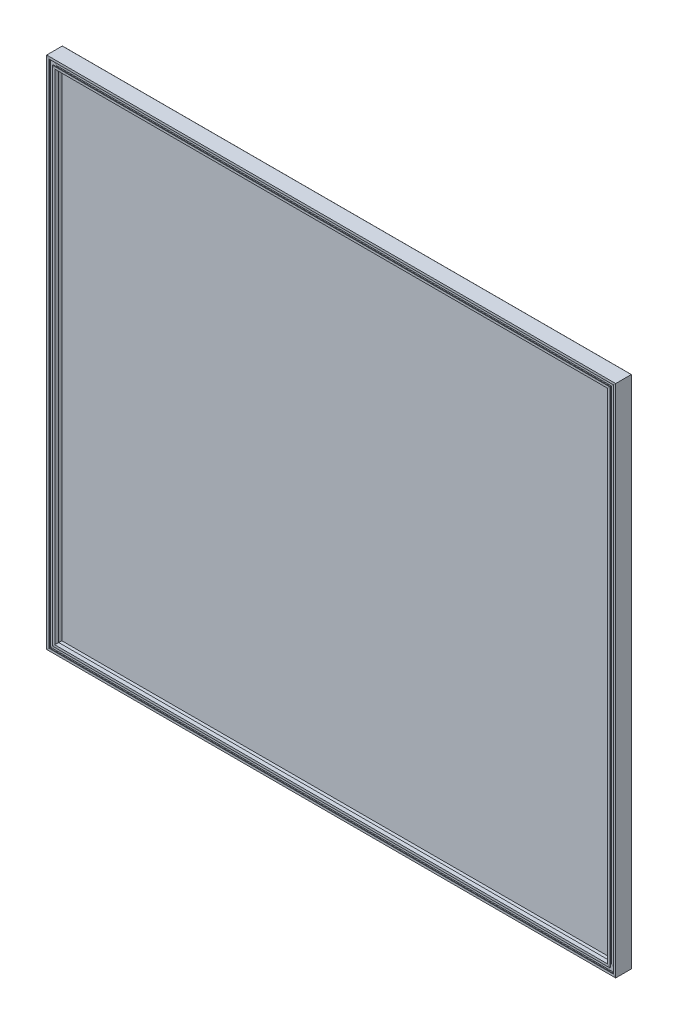
from build123d import *

# Parameters (mm, degrees)
MEMBER_1_DEPTH      = 40.357337308
MEMBER_1_DEPTH_BACK = 1300.357337308
MEMBER_1_2_DEPTH    = 1220.714674617
MEMBER_1_3_DEPTH    = 1340.714674617
MEMBER_1_4_DEPTH    = 1220.714674617
SKETCH_12_W         = 1250
SKETCH_12_H         = 1130
EXTRUDE_1_DEPTH     = 3


with BuildPart() as part:
    # 草图11 → Member 1 (new, two sides: drawn at the far end of the back side and taken through both)
    with BuildSketch(Plane(origin=(-630, 570, 0), x_dir=(0, -1, 0), z_dir=(-1, 0, 0)).offset(-MEMBER_1_DEPTH_BACK)):
        with BuildLine():
            Line((13, -1.5), (13, 0))
            Line((13, 0), (18, 0))
            Line((18, 0), (18, -8.7))
            Line((18, -8.7), (2, -8.7))
            Line((2, -8.7), (2, -32))
            ThreePointArc((2, -32), (2.292893219, -32.707106781), (3, -33))
            Line((3, -33), (8, -33))
            Line((8, -33), (8, -31.5))
            Line((8, -31.5), (10, -31.5))
            Line((10, -31.5), (10, -35))
            Line((10, -35), (0.5, -35))
            ThreePointArc((0.5, -35), (0.146446609, -34.853553391), (0, -34.5))
            Line((0, -34.5), (0, 0))
            Line((0, 0), (5, 0))
            Line((5, 0), (5, -1.5))
            Line((5, -1.5), (2, -1.5))
            Line((2, -1.5), (2, -6.7))
            Line((2, -6.7), (16, -6.7))
            Line((16, -6.7), (16, -1.5))
            Line((16, -1.5), (13, -1.5))
        make_face()
    extrude(amount=MEMBER_1_DEPTH + MEMBER_1_DEPTH_BACK)

    # Member 1 mitre 1
    split(bisect_by=Plane(origin=(-630, 570, 0), x_dir=(-0.707106781, 0.707106781, 0), z_dir=(0.707106781, 0.707106781, 0)), keep=Keep.TOP)

    # Member 1 mitre 2
    split(bisect_by=Plane(origin=(630, 570, 0), x_dir=(-0.707106781, -0.707106781, 0), z_dir=(-0.707106781, 0.707106781, 0)), keep=Keep.TOP)


with BuildPart() as body_2:
    # 草图11 on segment 2 (carried to segment 2) → Member 1 2 (new body)
    with BuildSketch(Plane(origin=(630, -610.357337308, 0), x_dir=(-1, 0, 0), z_dir=(0, 1, 0))):
        with BuildLine():
            Line((13, -1.5), (13, 0))
            Line((13, 0), (18, 0))
            Line((18, 0), (18, -8.7))
            Line((18, -8.7), (2, -8.7))
            Line((2, -8.7), (2, -32))
            ThreePointArc((2, -32), (2.292893219, -32.707106781), (3, -33))
            Line((3, -33), (8, -33))
            Line((8, -33), (8, -31.5))
            Line((8, -31.5), (10, -31.5))
            Line((10, -31.5), (10, -35))
            Line((10, -35), (0.5, -35))
            ThreePointArc((0.5, -35), (0.146446609, -34.853553391), (0, -34.5))
            Line((0, -34.5), (0, 0))
            Line((0, 0), (5, 0))
            Line((5, 0), (5, -1.5))
            Line((5, -1.5), (2, -1.5))
            Line((2, -1.5), (2, -6.7))
            Line((2, -6.7), (16, -6.7))
            Line((16, -6.7), (16, -1.5))
            Line((16, -1.5), (13, -1.5))
        make_face()
    extrude(amount=MEMBER_1_2_DEPTH)

    # Member 1 2 mitre 1
    split(bisect_by=Plane(origin=(630, 570, 0), x_dir=(0.707106781, 0.707106781, 0), z_dir=(0.707106781, -0.707106781, 0)), keep=Keep.TOP)

    # Member 1 2 mitre 2
    split(bisect_by=Plane(origin=(630, -570, 0), x_dir=(-0.707106781, 0.707106781, 0), z_dir=(0.707106781, 0.707106781, 0)), keep=Keep.TOP)


with BuildPart() as body_3:
    # 草图11 on segment 3 (carried to segment 3) → Member 1 3 (new body)
    with BuildSketch(Plane(origin=(-670.357337308, -570, 0), x_dir=(0, 1, 0), z_dir=(1, 0, 0))):
        with BuildLine():
            Line((13, -1.5), (13, 0))
            Line((13, 0), (18, 0))
            Line((18, 0), (18, -8.7))
            Line((18, -8.7), (2, -8.7))
            Line((2, -8.7), (2, -32))
            ThreePointArc((2, -32), (2.292893219, -32.707106781), (3, -33))
            Line((3, -33), (8, -33))
            Line((8, -33), (8, -31.5))
            Line((8, -31.5), (10, -31.5))
            Line((10, -31.5), (10, -35))
            Line((10, -35), (0.5, -35))
            ThreePointArc((0.5, -35), (0.146446609, -34.853553391), (0, -34.5))
            Line((0, -34.5), (0, 0))
            Line((0, 0), (5, 0))
            Line((5, 0), (5, -1.5))
            Line((5, -1.5), (2, -1.5))
            Line((2, -1.5), (2, -6.7))
            Line((2, -6.7), (16, -6.7))
            Line((16, -6.7), (16, -1.5))
            Line((16, -1.5), (13, -1.5))
        make_face()
    extrude(amount=MEMBER_1_3_DEPTH)

    # Member 1 3 mitre 1
    split(bisect_by=Plane(origin=(-630, -570, 0), x_dir=(0.707106781, 0.707106781, 0), z_dir=(0.707106781, -0.707106781, 0)), keep=Keep.TOP)

    # Member 1 3 mitre 2
    split(bisect_by=Plane(origin=(630, -570, 0), x_dir=(0.707106781, -0.707106781, 0), z_dir=(-0.707106781, -0.707106781, 0)), keep=Keep.TOP)


with BuildPart() as body_4:
    # 草图11 on segment 4 (carried to segment 4) → Member 1 4 (new body)
    with BuildSketch(Plane(origin=(-630, 610.357337308, 0), x_dir=(1, 0, 0), z_dir=(0, -1, 0))):
        with BuildLine():
            Line((13, -1.5), (13, 0))
            Line((13, 0), (18, 0))
            Line((18, 0), (18, -8.7))
            Line((18, -8.7), (2, -8.7))
            Line((2, -8.7), (2, -32))
            ThreePointArc((2, -32), (2.292893219, -32.707106781), (3, -33))
            Line((3, -33), (8, -33))
            Line((8, -33), (8, -31.5))
            Line((8, -31.5), (10, -31.5))
            Line((10, -31.5), (10, -35))
            Line((10, -35), (0.5, -35))
            ThreePointArc((0.5, -35), (0.146446609, -34.853553391), (0, -34.5))
            Line((0, -34.5), (0, 0))
            Line((0, 0), (5, 0))
            Line((5, 0), (5, -1.5))
            Line((5, -1.5), (2, -1.5))
            Line((2, -1.5), (2, -6.7))
            Line((2, -6.7), (16, -6.7))
            Line((16, -6.7), (16, -1.5))
            Line((16, -1.5), (13, -1.5))
        make_face()
    extrude(amount=MEMBER_1_4_DEPTH)

    # Member 1 4 mitre 1
    split(bisect_by=Plane(origin=(-630, 570, 0), x_dir=(0.707106781, -0.707106781, 0), z_dir=(-0.707106781, -0.707106781, 0)), keep=Keep.TOP)

    # Member 1 4 mitre 2
    split(bisect_by=Plane(origin=(-630, -570, 0), x_dir=(-0.707106781, -0.707106781, 0), z_dir=(-0.707106781, 0.707106781, 0)), keep=Keep.TOP)


with BuildPart() as body_5:
    # 草图12 → 凸台-拉伸1 (new body)
    with BuildSketch(Plane.XY.offset(-31.5)):
        Rectangle(SKETCH_12_W, SKETCH_12_H)
    extrude(amount=EXTRUDE_1_DEPTH)


solid = Compound([part.part, body_2.part, body_3.part, body_4.part, body_5.part])
